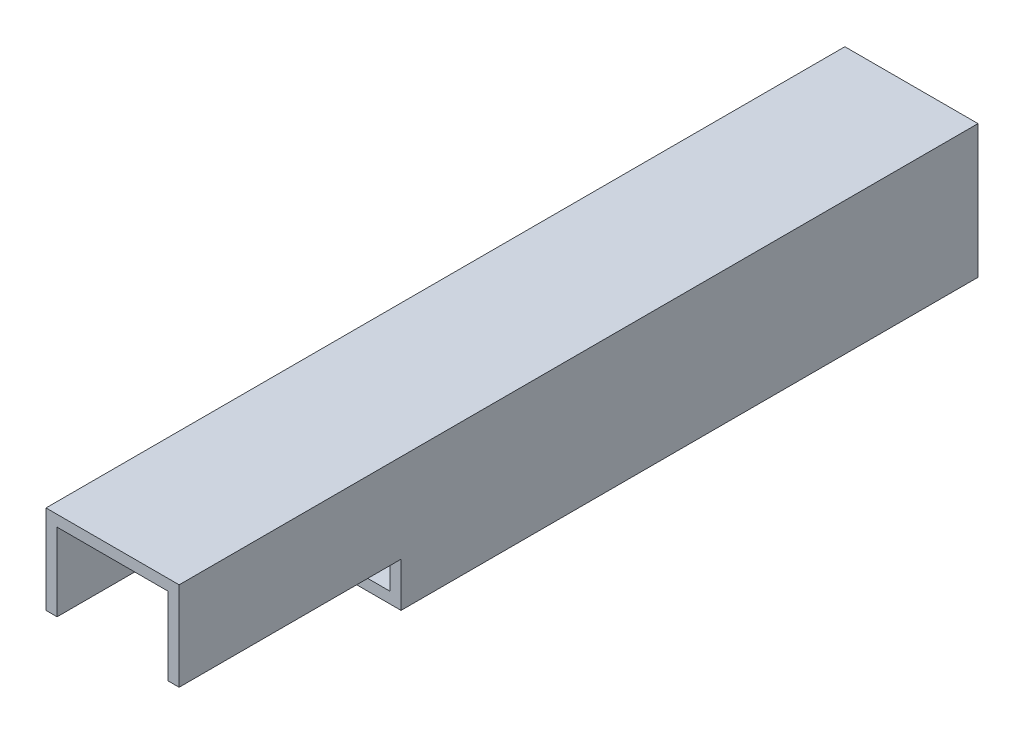
from build123d import *

# Parameters (mm, degrees)
SKETCH1_W               = 30
SKETCH1_H               = 30
BOSS_EXTRUDE1_DEPTH     = 180
SKETCH5_W               = 25
SKETCH5_H               = 25
CUT_EXTRUDE4_DEPTH      = 182.245689604
CUT_EXTRUDE3_DEPTH      = 184.098334236
CUT_EXTRUDE3_DEPTH_BACK = 10


with BuildPart() as part:
    # Sketch1 → Boss-Extrude1 (new body)
    with BuildSketch(Plane.XY):
        Rectangle(SKETCH1_W, SKETCH1_H)
    extrude(amount=BOSS_EXTRUDE1_DEPTH)

    # Sketch5 → Cut-Extrude4 (cut, through all)
    with BuildSketch(Plane(origin=(0, 0, 0), x_dir=(-1, 0, 0), z_dir=(0, 0, -1))):
        Rectangle(SKETCH5_W, SKETCH5_H)
    extrude(amount=-CUT_EXTRUDE4_DEPTH, mode=Mode.SUBTRACT)

    # Sketch3 → Cut-Extrude3 (cut, two sides: drawn at the far end of the back side and taken through both)
    with BuildSketch(Plane.XZ.offset(15).offset(-CUT_EXTRUDE3_DEPTH_BACK)):
        Polygon((-389.965751818, 130), (-15, 130), (15, 130), (15, 180), (15, 554.965751818), (-527.902959777, 1072.318278062), (-932.868711595, 647.352526244), align=None)
    extrude(amount=CUT_EXTRUDE3_DEPTH + CUT_EXTRUDE3_DEPTH_BACK, mode=Mode.SUBTRACT)


solid = part.part
